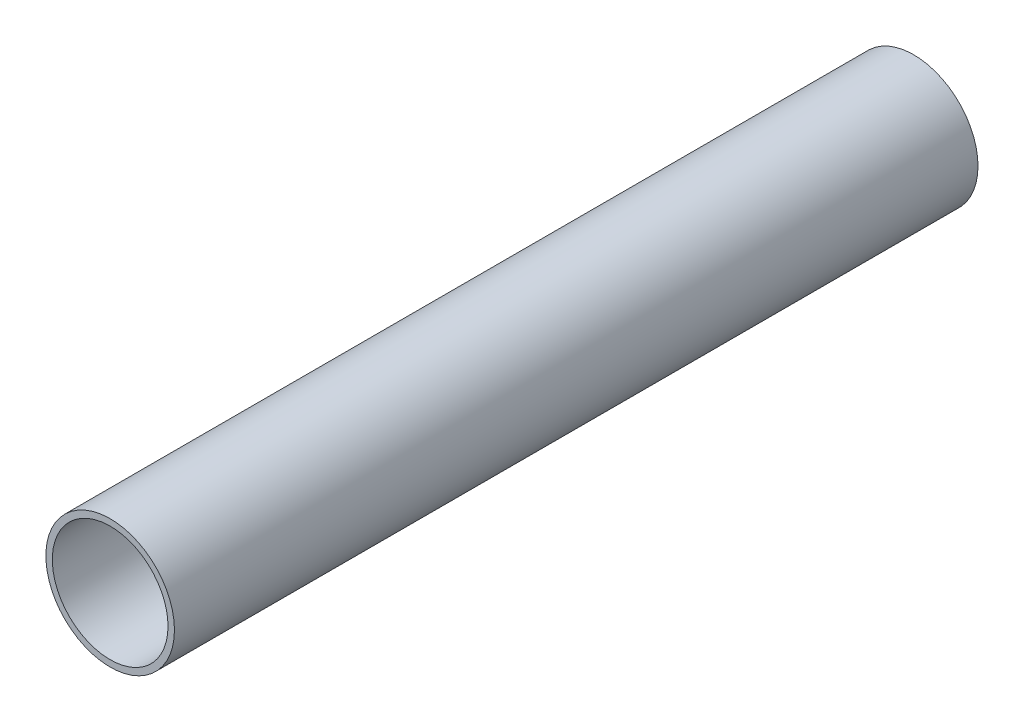
SolidWorks part; units mm, degrees
ref_plane "前视基准面" through (0, 0, 0) normal (0, 0, 1) x (1, 0, 0)
ref_plane "上视基准面" through (0, 0, 0) normal (0, 1, 0) x (1, 0, 0)
ref_plane "右视基准面" through (0, 0, 0) normal (1, 0, 0) x (0, 0, -1)
sketch "草图1" plane through (0, 0, 0) normal (0, 0, 1) x (1, 0, 0)
  circle A0 centre (0, 0) radius 20
  circle A1 centre (0, 0) radius 18
  dimension "D1" = 2
extrude "凸台-拉伸1" add sketch "草图1" along normal blind 250
